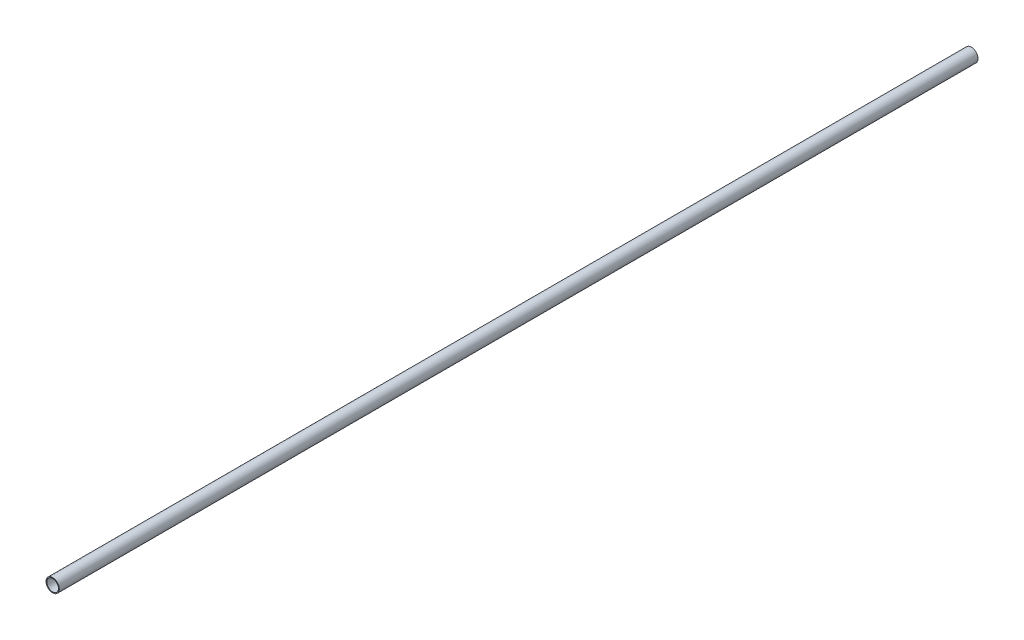
SolidWorks part; units mm, degrees
ref_plane "前视基准面" through (0, 0, 0) normal (0, 0, 1) x (1, 0, 0)
ref_plane "上视基准面" through (0, 0, 0) normal (0, 1, 0) x (1, 0, 0)
ref_plane "右视基准面" through (0, 0, 0) normal (1, 0, 0) x (0, 0, -1)
sketch "草图1" plane through (0, 0, 0) normal (0, 0, 1) x (1, 0, 0)
  circle A0 centre (0, 0) radius 16
  circle A1 centre (0, 0) radius 14
  dimension "D1" = 32
  dimension "D2" = 2
extrude "凸台-拉伸1" add sketch "草图1" along normal mid plane 2210
sketch "草图2" plane through (0, 0, -1105) normal (0, 0, -1) x (-1, 0, 0)
  line L0 (0, 0) -> (16, 0)
  circle A0 centre (0, 0) radius 16 construction
